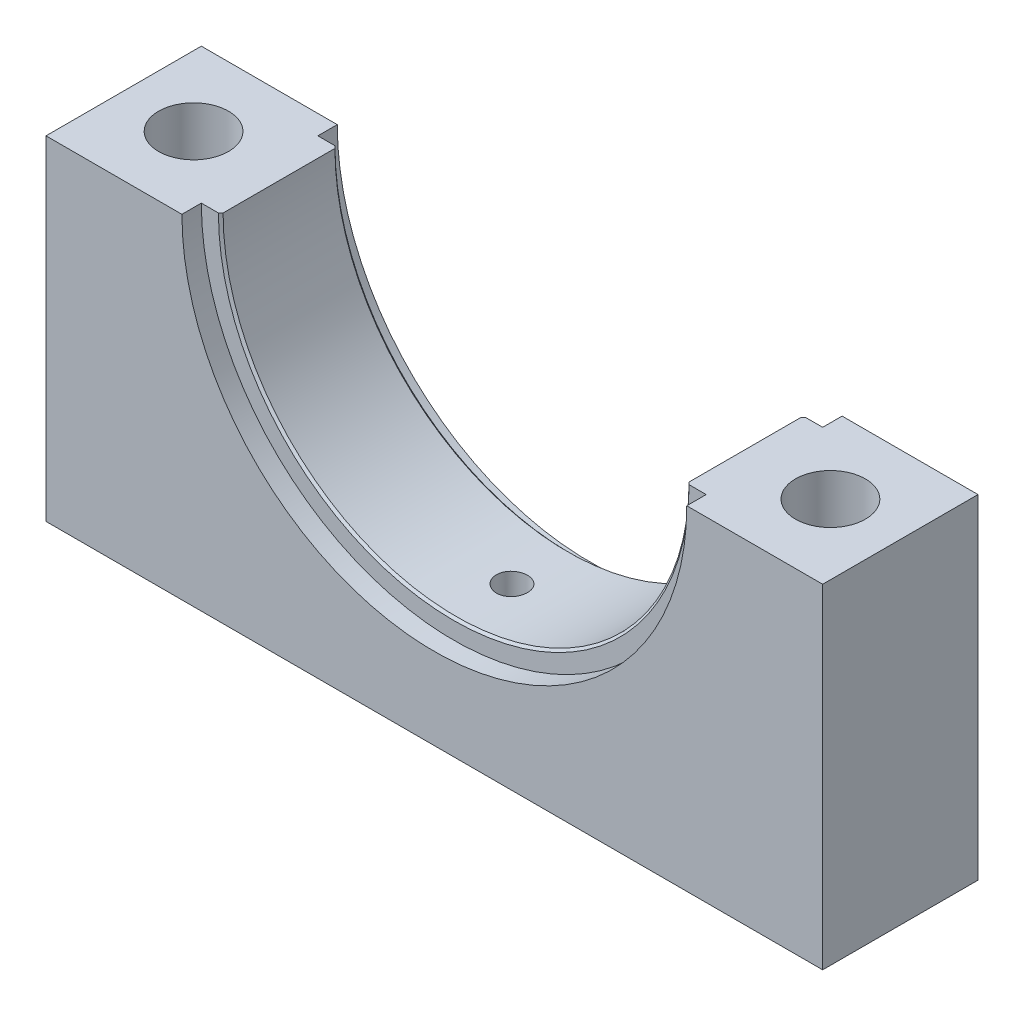
SolidWorks part; units mm, degrees
material "Q235-A"
ref_plane "Front Plane" through (0, 0, 0) normal (0, 0, 1) x (1, 0, 0)
ref_plane "Top Plane" through (0, 0, 0) normal (0, 1, 0) x (1, 0, 0)
ref_plane "Right Plane" through (0, 0, 0) normal (1, 0, 0) x (0, 0, -1)
sketch "Sketch1" plane through (0, 0, 0) normal (0, 0, 1) x (1, 0, 0)
  line L0 (-50, 0) -> (-30, 0)
  line L1 (-50, -43) -> (50, -43)
  line L2 (-50, -43) -> (-50, 0)
  line L4 (50, -43) -> (50, 0)
  line L5 (-50, -43) -> (0, 0) construction
  line L6 (22.7456, -19.5612) -> (50, -43) construction
  line L7 (30, 0) -> (50, 0)
  arc A0 (-30, 0) -> (30, 0) centre (0, 0) ccw
  point P0 (0, 0)
  dimension "D1" = 43
  dimension "D2" = 100
extrude "Boss-Extrude1" add sketch "Sketch1" along normal blind 20
sketch "Sketch2" plane through (0, 0, 20) normal (0, 0, 1) x (1, 0, 0)
  circle A0 centre (0, 0) radius 32.5
extrude "Cut-Extrude1" cut sketch "Sketch2" against normal blind 2.5
sketch "Sketch3" plane through (0, 0, 0) normal (0, 0, -1) x (-1, 0, 0)
  circle A1 centre (0, 0) radius 32.5
  circle A2 centre (0, 0) radius 32.5
  dimension "D1" = 0
extrude "Cut-Extrude2" cut sketch "Sketch3" against normal blind 2.5
chamfer "Chamfer1" distance 0.3 angle 45 2 edges at (0, -30, 2.5) (0, -30, 17.5)
sketch "Sketch4" plane through (0, 0, 0) normal (0, 1, 0) x (1, 0, 0)
  line L0 (-41, -10) -> (41, -10)
  line L1 (-50, -20) -> (-50, 0) construction
  line L2 (50, 0) -> (32.5, 0) construction
  dimension "D1" = 82
  dimension "D2" = 9
  dimension "D3" = 10
hole_wizard "Hole1" positions "Sketch5" profile "Sketch6" legacy end condition through all
sketch "Sketch5" plane through (0, 0, 0) normal (0, 1, 0) x (1, 0, 0)
  point P0 (-41, -10)
  point P3 (41, -10)
sketch "Sketch6" plane through (-41, 0, 10) normal (1, 0, 0) x (0, 0, 1)
  line L0 (0, 0) -> (0, 43)
  line L1 (0, 43) -> (4.5, 43)
  line L2 (4.5, 43) -> (4.5, 0)
  line L3 (4.5, 0) -> (0, 0)
  line L4 (0, 110) -> (0, -10) construction
  dimension "直径" = 9
  dimension "深度" = 43
sketch "Sketch8" plane through (0, 0, 0) normal (0, 1, 0) x (1, 0, 0)
  line L0 (0, -20) -> (0, 0)
  line L1 (-32.5, -20) -> (32.5, -20) construction
  line L2 (32.5, 0) -> (-32.5, 0) construction
hole_wizard "Hole2" positions "Sketch9" profile "Sketch10" legacy
sketch "Sketch9" plane through (0, 0, 0) normal (0, 1, 0) x (1, 0, 0)
  line L0 (0, -20) -> (0, 0) construction
  point P0 (0, -10)
sketch "Sketch10" plane through (0, 0, 10) normal (1, 0, 0) x (0, 0, 1)
  line L0 (0, 0) -> (0, 34)
  line L1 (0, 34) -> (2, 34)
  line L2 (2, 34) -> (2, 0)
  line L3 (2, 0) -> (0, 0)
  line L4 (0, 110) -> (0, -10) construction
  dimension "直径" = 4
  dimension "深度" = 34
